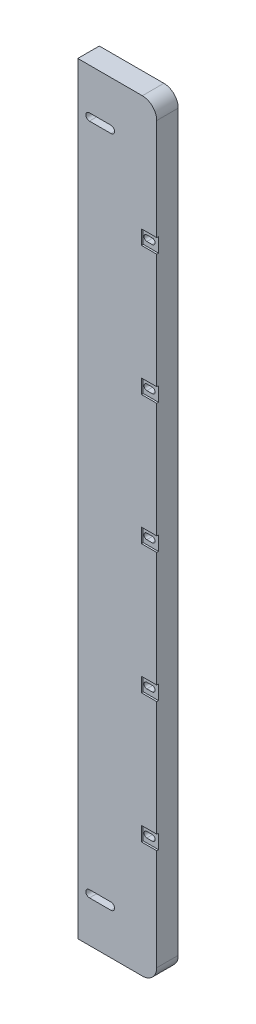
SolidWorks part; units mm, degrees
ref_plane "前视基准面" through (0, 0, 0) normal (0, 0, 1) x (1, 0, 0)
ref_plane "上视基准面" through (0, 0, 0) normal (0, 1, 0) x (1, 0, 0)
ref_plane "右视基准面" through (0, 0, 0) normal (1, 0, 0) x (0, 0, -1)
sketch "草图1" plane through (0, 0, 0) normal (0, 0, 1) x (1, 0, 0)
  line L1 (22, 212.5) -> (-22, 212.5)
  line L2 (22, 212.5) -> (22, -212.5)
  line L3 (22, -212.5) -> (-22, -212.5)
  line L4 (-22, 212.5) -> (-22, -212.5)
  line L5 (22, 212.5) -> (-22, -212.5) construction
  line L6 (22, -212.5) -> (-22, 212.5) construction
  point P0 (0, 0)
  dimension "D1" = 44
  dimension "D2" = 425
extrude "凸台-拉伸1" add sketch "草图1" along normal blind 12
fillet "圆角1" radius 8 2 edges at (22, 212.5, 6) (22, -212.5, 6)
sketch "草图3" plane through (0, 0, 0) normal (0, 0, -1) x (-1, 0, 0)
  line L0 (3.5, 187.5) -> (15.5, 187.5) construction
  line L1 (3.5, 191.5) -> (15.5, 191.5)
  line L2 (3.5, 183.5) -> (15.5, 183.5)
  line L3 (22, 212.5) -> (22, -212.5) construction
  line L4 (-14, 212.5) -> (22, 212.5) construction
  line L5 (32.5187, 0) -> (-33.7363, 0) construction
  line L6 (3.5, -187.5) -> (15.5, -187.5) construction
  line L7 (3.5, -191.5) -> (15.5, -191.5)
  line L8 (3.5, -183.5) -> (15.5, -183.5)
  arc A0 (3.5, 191.5) -> (3.5, 183.5) centre (3.5, 187.5) ccw
  arc A1 (15.5, 183.5) -> (15.5, 191.5) centre (15.5, 187.5) ccw
  arc A2 (3.5, -191.5) -> (3.5, -183.5) centre (3.5, -187.5) cw
  arc A3 (15.5, -183.5) -> (15.5, -191.5) centre (15.5, -187.5) cw
  point P2 (9.5, 187.5)
  point P16 (9.5, -187.5)
  dimension "D4" = 4
  dimension "D1" = 12
  dimension "D2" = 6.5
  dimension "D3" = 25
extrude "切除-拉伸1" cut sketch "草图3" against normal blind 6
sketch "草图4" plane through (0, 0, 6) normal (0, 0, -1) x (-1, 0, 0)
  line L0 (3.5, 187.5) -> (15.5, 187.5) construction
  line L1 (3.5, 189.5) -> (15.5, 189.5)
  line L2 (3.5, 185.5) -> (15.5, 185.5)
  line L3 (29.2983, 0) -> (-30.2191, 0) construction
  line L4 (3.5, -187.5) -> (15.5, -187.5) construction
  line L5 (3.5, -189.5) -> (15.5, -189.5)
  line L6 (3.5, -185.5) -> (15.5, -185.5)
  arc A0 (3.5, 189.5) -> (3.5, 185.5) centre (3.5, 187.5) ccw
  arc A1 (15.5, 185.5) -> (15.5, 189.5) centre (15.5, 187.5) ccw
  arc A2 (3.5, -189.5) -> (3.5, -185.5) centre (3.5, -187.5) cw
  arc A3 (15.5, -185.5) -> (15.5, -189.5) centre (15.5, -187.5) cw
  point P4 (9.5, 187.5)
  point P14 (9.5, -187.5)
  dimension "D1" = 2
extrude "切除-拉伸2" cut sketch "草图4" against normal through all
sketch "草图6" plane through (0, 0, 12) normal (0, 0, 1) x (1, 0, 0)
  line L0 (22, -204.5) -> (22, 204.5) construction
  line L1 (22, 148) -> (13.5, 148)
  line L2 (22, 148) -> (22, 140)
  line L3 (22, 140) -> (13.5, 140)
  line L4 (13.5, 148) -> (13.5, 140)
  line L5 (14, 212.5) -> (-22, 212.5) construction
  line L6 (22, 76) -> (13.5, 76)
  line L7 (22, 76) -> (22, 68)
  line L8 (22, 68) -> (13.5, 68)
  line L9 (13.5, 76) -> (13.5, 68)
  line L10 (22, 4) -> (13.5, 4)
  line L11 (22, 4) -> (22, -4)
  line L12 (22, -4) -> (13.5, -4)
  line L13 (13.5, 4) -> (13.5, -4)
  line L14 (22, -68) -> (13.5, -68)
  line L15 (22, -68) -> (22, -76)
  line L16 (22, -76) -> (13.5, -76)
  line L17 (13.5, -68) -> (13.5, -76)
  line L18 (22, -140) -> (13.5, -140)
  line L19 (22, -140) -> (22, -148)
  line L20 (22, -148) -> (13.5, -148)
  line L21 (13.5, -140) -> (13.5, -148)
  dimension "D1" = 64.5
  dimension "D2" = 8
  dimension "D3" = 8.5
extrude "切除-拉伸4" cut sketch "草图6" against normal blind 1
sketch "草图7" plane through (0, 0, 0) normal (0, 0, -1) x (-1, 0, 0)
  line L0 (-18.5, 144) -> (-15.5, 144) construction
  line L1 (-18.5, 147) -> (-15.5, 147)
  line L2 (-18.5, 141) -> (-15.5, 141)
  line L3 (-14, 212.5) -> (22, 212.5) construction
  line L4 (-22, -204.5) -> (-22, 204.5) construction
  arc A0 (-18.5, 147) -> (-18.5, 141) centre (-18.5, 144) ccw
  arc A1 (-15.5, 141) -> (-15.5, 147) centre (-15.5, 144) ccw
  point P2 (-17, 144)
  dimension "D3" = 3
  dimension "D1" = 68.5
  dimension "D2" = 3.5
  dimension "D4" = 3
extrude "切除-拉伸5" cut sketch "草图7" against normal blind 4
sketch "草图8" plane through (0, 0, 4) normal (0, 0, -1) x (-1, 0, 0)
  line L0 (-18.5, 144) -> (-15.5, 144) construction
  line L1 (-18.5, 145.6) -> (-15.5, 145.6)
  line L2 (-18.5, 142.4) -> (-15.5, 142.4)
  arc A0 (-18.5, 145.6) -> (-18.5, 142.4) centre (-18.5, 144) ccw
  arc A1 (-15.5, 142.4) -> (-15.5, 145.6) centre (-15.5, 144) ccw
  point P4 (-17, 144)
  dimension "D1" = 1.6
extrude "切除-拉伸6" cut sketch "草图8" against normal through all
pattern_linear "阵列(线性)1" count 5 spacing 72 along (0, -1, 0) of "切除-拉伸5", "切除-拉伸6"
